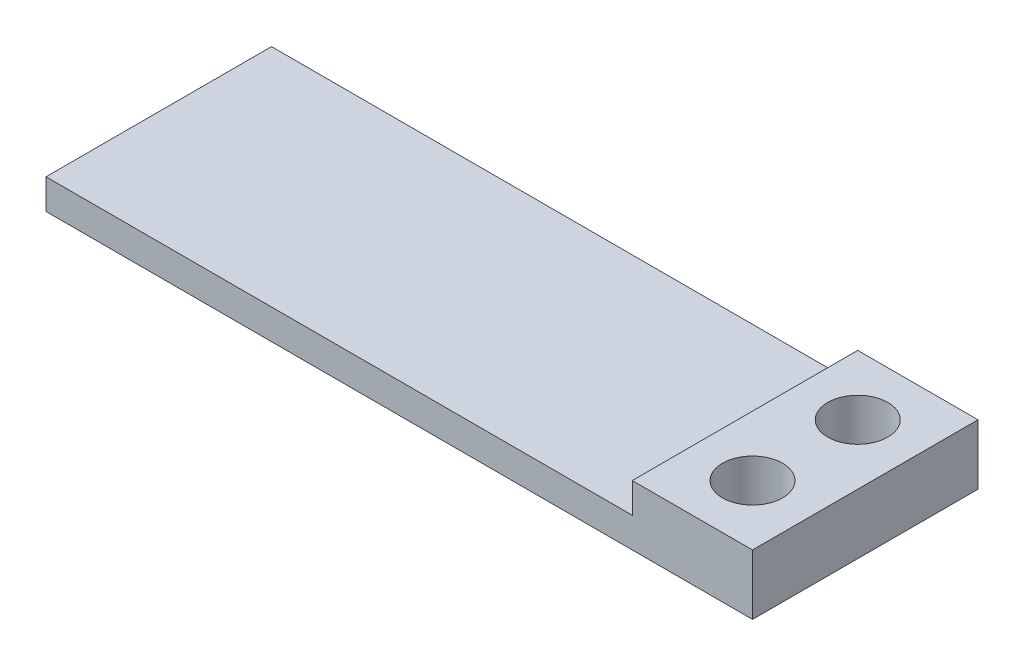
SolidWorks part; units mm, degrees
ref_plane "前视基准面" through (0, 0, 0) normal (0, 0, 1) x (1, 0, 0)
ref_plane "上视基准面" through (0, 0, 0) normal (0, 1, 0) x (1, 0, 0)
ref_plane "右视基准面" through (0, 0, 0) normal (1, 0, 0) x (0, 0, -1)
sketch "草图1" plane through (0, 0, 0) normal (0, 0, 1) x (1, 0, 0)
  line L0 (0, 0) -> (47, 0)
  line L1 (47, 0) -> (47, 4)
  line L2 (47, 4) -> (39, 4)
  line L3 (39, 4) -> (39, 2)
  line L4 (39, 2) -> (0, 2)
  line L5 (0, 2) -> (0, 0)
  dimension "D1" = 2
  dimension "D2" = 2
  dimension "D3" = 8
  dimension "D4" = 39
extrude "凸台-拉伸1" add sketch "草图1" along normal mid plane 15
sketch "草图2" plane through (0, 4, 0) normal (0, 1, 0) x (1, 0, 0)
  line L0 (47, 7.5) -> (39, 7.5) construction
  line L1 (47, -7.5) -> (39, -7.5) construction
  line L2 (47, -7.5) -> (47, 7.5) construction
  circle A0 centre (43, 3.5) radius 2
  circle A1 centre (43, -3.5) radius 2
  dimension "D1" = 4
  dimension "D2" = 4
  dimension "D3" = 4
  dimension "D4" = 4
extrude "切除-拉伸1" cut sketch "草图2" against normal up to next
